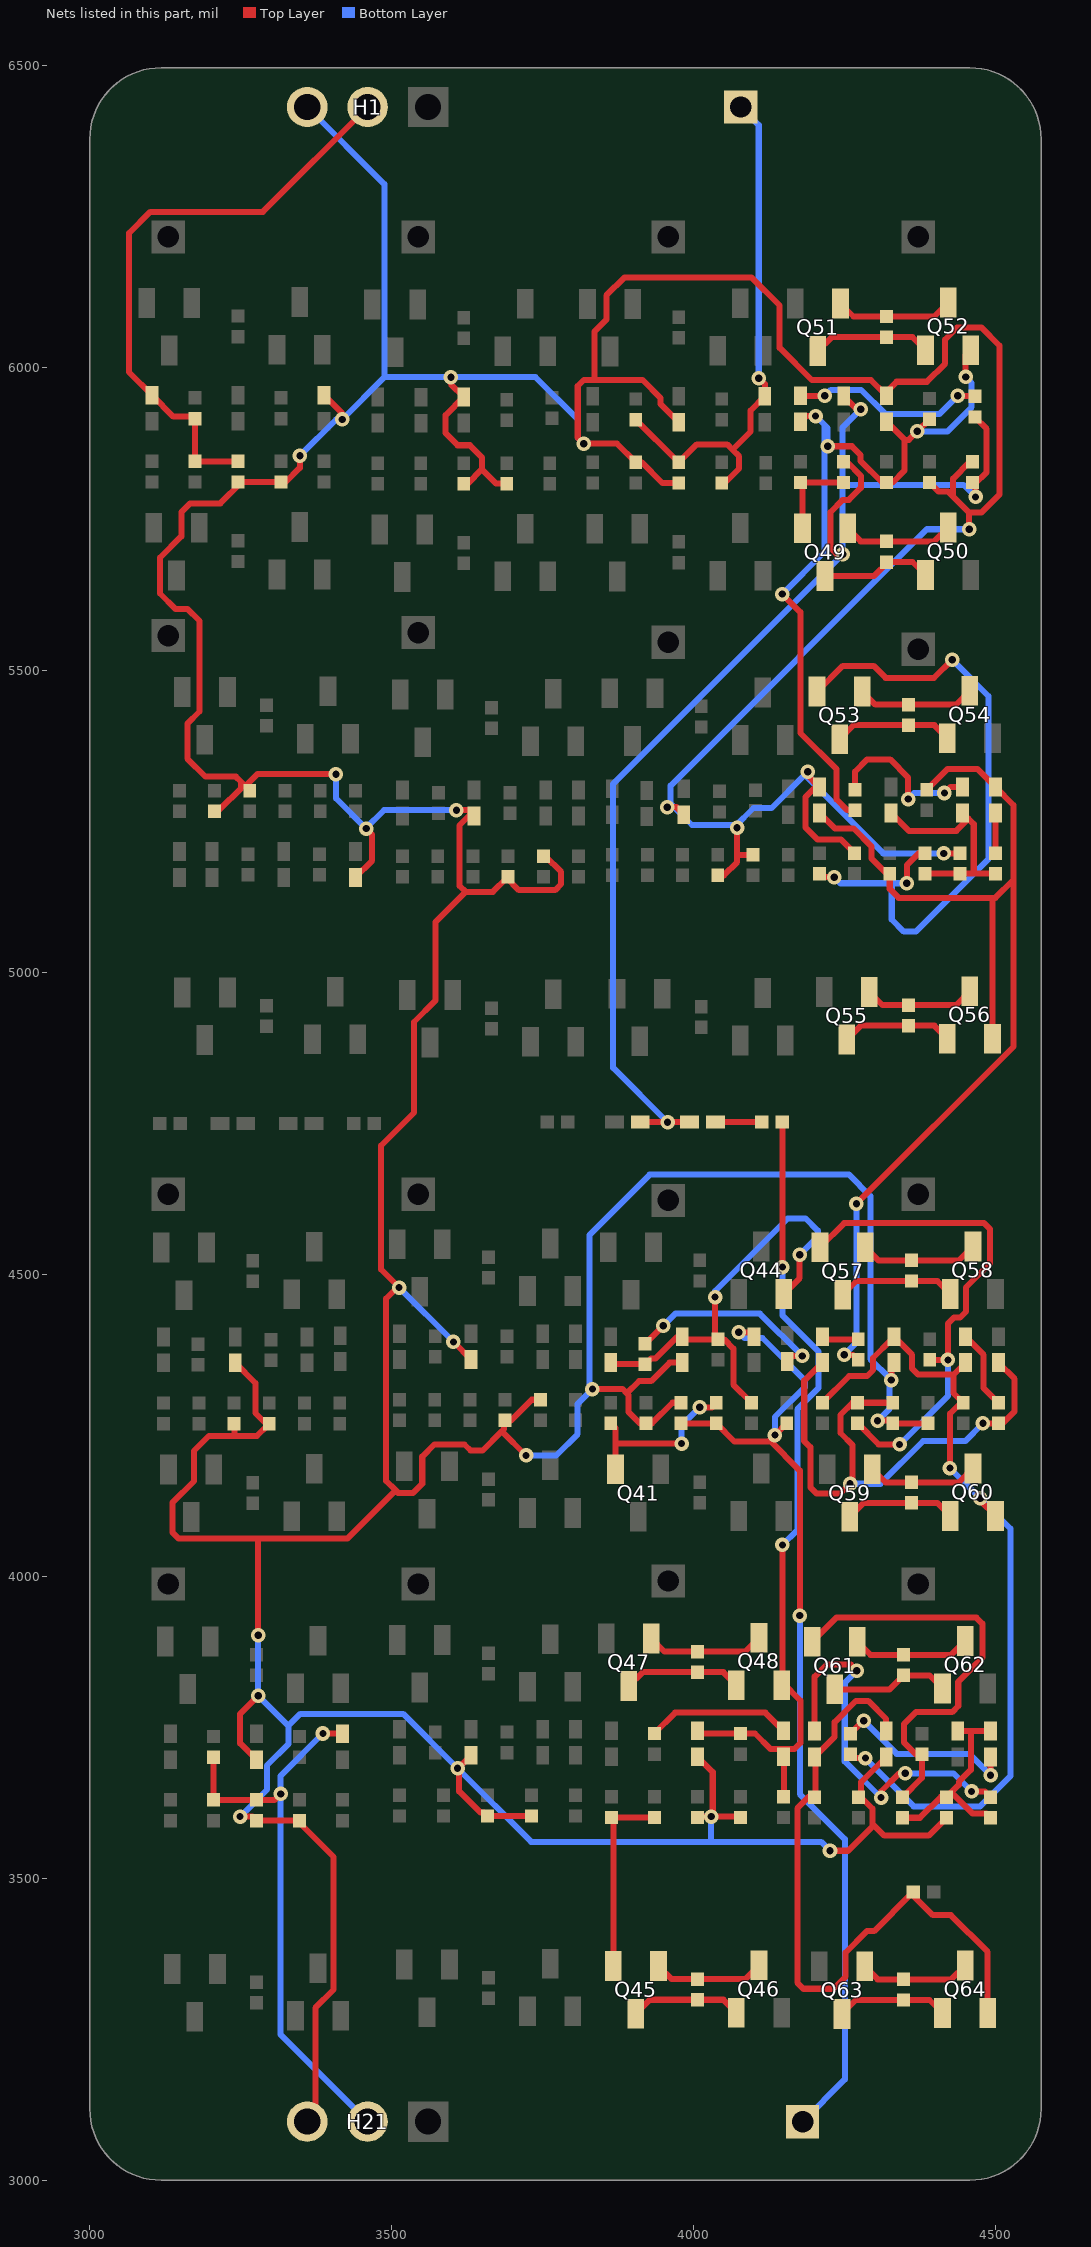
[diagram p0: the nets of this part, all layers, seen from the top]
# Altium PCB MISC61260.pcbdoc (part 3 of 4)
Units mil, origin at the board's own origin, x right, y up, seen from the top; angles counter-clockwise.
Board outline 1574.8 x 3497.01 mil, 2 copper layers (Top Layer, Bottom Layer), stack 62.206 mil thick; 303 components, 159 nets, 654 pads, 177 vias.

## Via types
v1: diameter 24.02, hole 12, Top Layer to Bottom Layer, 177 vias

## Nets (pads, with @x,y where several pads share a name; then routed paths per layer and width w, separated by ;. In a path a pad name is that pad's centre, name@x,y a point inside that pad or via, vN(x,y) a via of type N, cw(c..) or ccw(c..) an arc to the next point about the centre after c; other vN are vias at no path point) (continued)
$1N11454: C44.2 R42.1 | length 338.2
  Top Layer w10: R42.1@3919.35,4384.53 v1(3949.35,4414.53) ; C44.2@4154.58,4355.55 4163.56,4364.53 v1(4179.35,4364.53)
  Bottom Layer w10: v1(3949.35,4414.53) 3969.35,4434.53 4109.35,4434.53 v1(4179.35,4364.53)
$1N11455: C42.1 C43.1 Q44.2 R42.2 R43.2 Rp22.1 | length 771.1
  Top Layer w10: C43.1@3862.33,4353.53 3864.49,4351.37 R42.2@3920.28,4351.37 ; R42.2@3919.35,4350.45 R42.2@3920.28,4351.37 ; C42.1@3980.89,4396.45 C42.1@3981.78,4395.57 ; v1(4035.17,4462.03) Rp22.1@4035.17,4392.03 ; R43.2@4095.45,4287.03 4065.45,4317.03 4065.45,4376.75 4050.17,4392.03 Rp22.1@4040.17,4392.03 Rp22.1@4035.17,4392.03 ; Q44.2@4148.98,4467 4175.17,4493.19 v1(4175.17,4532.03) ; R42.2@3920.28,4351.37 3929.11,4360.21 3936.42,4360.21 3971.78,4395.57 C42.1@3981.78,4395.57 ; C42.1@3981.78,4395.57 3985.31,4392.03 Rp22.1@4035.17,4392.03
  Bottom Layer w10: v1(4035.17,4462.03) 4035.17,4472.03 4155.17,4592.03 4185.17,4592.03 4205.17,4572.03 4205.17,4562.03 v1(4175.17,4532.03)
$1N11457: Q41.2 Rp21.2 Rs21.1 | length 291.6
  Top Layer w10: Rp21.2@3862.33,4252.95 3870.39,4244.89 3870.39,4219.51 ; Q41.2@3870.39,4177.01 3870.39,4219.51 ; v1(3979.65,4219.51) 3870.39,4219.51 ; v1(4009.65,4279.51) 4029.65,4279.51 Rs21.1@4037.17,4287.03
  Bottom Layer w10: v1(3979.65,4219.51) 3979.65,4249.51 v1(4009.65,4279.51)
$1N11459: Q45.3 Q46.1 Rb23.2 | length 184.9
  Top Layer w10: Q45.3@3904.06,3275.77 3927.08,3298.79 Rb23.2@4005.95,3298.79 4048.81,3298.79 Q46.1@4070.45,3277.15
$1N11460: Q45.1 Q46.3 Rb23.1 | length 184.9
  Top Layer w10: Q45.1@3941.46,3354.51 3963.1,3332.87 Rb23.1@4005.95,3332.87 4084.83,3332.87 Q46.3@4107.85,3355.89
$1N11461: Q45.2 Rp23.2 Rs23.1 | length 318.4
  Top Layer w10: Q45.2@3866.66,3354.51 3866.66,3597.39 Rp23.2@3863.6,3600.45 Rs23.1@3934.78,3600.45
$1N11462: Q47.3 Q48.1 Rb24.2 | length 196.8
  Top Layer w10: Q47.3@3892.15,3818.12 3915.17,3841.14 Rb24.2@4005.95,3841.14 4048.81,3841.14 Q48.1@4070.45,3819.5
$1N11463: Q47.1 Q48.3 Rb24.1 | length 196.8
  Top Layer w10: Q47.1@3929.55,3896.86 3951.19,3875.22 Rb24.1@4005.95,3875.22 4084.83,3875.22 Q48.3@4107.85,3898.24
$1N11464: C47.2 R45.1 | length 240.2
  Top Layer w10: R45.1@3934.78,3739.53 3969.2,3773.95 4118.31,3773.95 C47.2@4148.31,3743.95
$1N11466: C46.1 C47.1 Q48.2 R47.2 R48.2 Rp24.1 | length 1363
  Top Layer w10: C46.1@4005.95,3743.95 4010.37,3739.53 Rp24.1@4077.13,3739.53 4101.17,3739.53 4126.62,3714.09 C47.1@4149.12,3714.09 ; Q48.2@4145.25,3819.5 4146.62,3820.87 Q48.2@4146.62,3824.09 ; v1(4146.62,4051.59) Q48.2@4146.62,3824.09 ; v1(4146.62,4511.59) R48.2@4146.62,4751.59 ; R47.2@4148.31,3634.53 4149.12,3635.34 C47.1@4149.12,3701.84 ; C47.1@4148.31,3701.03 C47.1@4149.12,3701.84 ; Q48.2@4146.62,3824.09 4176.62,3794.09 4176.62,3724.09 4166.62,3714.09 C47.1@4149.12,3714.09 ; C47.1@4149.12,3701.84 C47.1@4149.12,3714.09
  Bottom Layer w10: v1(4146.62,4051.59) 4171.26,4076.23 4171.26,4276.23 4206.62,4311.59 4206.62,4371.59 4146.62,4431.59 v1(4146.62,4511.59)
$1N11467: C48.2 R48.1 | length 76.9
  Top Layer w10: C48.2@4035.65,4751.59 R48.1@4112.54,4751.59
$1N11468: C40.1 C48.1 C49.2 R49.2 R51.1 Rs25.2 | length 2096.7
  Top Layer w10: C40.1@3911.42,4751.59 v1(3956.42,4751.59) C48.1@3992.73,4751.59 ; v1(4246.42,5691.59) 4236.42,5691.59 4226.42,5701.59 4226.42,5761.59 4246.42,5781.59 4256.42,5781.59 4276.42,5801.59 4276.42,5821.59 4253.48,5844.53 Rs25.2@4247.91,5844.53 ; C49.2@4248.14,5953.47 4270.02,5931.59 v1(4276.42,5931.59) ; R51.1@4461.45,5810.45 R51.1@4464.66,5807.24 ; R49.2@4465.17,5918.87 4484.66,5899.38 4484.66,5827.24 R51.1@4464.66,5807.24 ; v1(4466.42,5786.59) 4466.42,5805.47 R51.1@4464.66,5807.24
  Bottom Layer w10: v1(3956.42,4751.59) 3866.42,4841.59 3866.42,5311.59 v1(4246.42,5691.59) 4246.42,5806.59 ; v1(4276.42,5931.59) 4246.42,5901.59 4246.42,5806.59 ; v1(4466.42,5786.59) 4446.42,5806.59 4246.42,5806.59
$1N11498: Q49.3 Q50.1 Rb25.2 | length 187.4
  Top Layer w10: Q49.3@4217.19,5655.77 4298.57,5655.77 Rb25.2@4321.59,5678.79 ; Rb25.2@4319.09,5678.79 Rb25.2@4321.59,5678.79 ; Q50.1@4383.59,5657.15 4361.95,5678.79 Rb25.2@4321.59,5678.79
$1N11499: Q49.1 Q50.3 Rb25.1 | length 184.9
  Top Layer w10: Q49.1@4254.59,5734.51 4276.23,5712.87 Rb25.1@4319.09,5712.87 4397.97,5712.87 Q50.3@4420.99,5735.89
$1N11500: Q51.3 Q52.1 Rb26.2 | length 196.8
  Top Layer w10: Q51.3@4205.29,6028.12 4228.31,6051.14 Rb26.2@4319.09,6051.14 4361.95,6051.14 Q52.1@4383.59,6029.5
$1N11501: Q51.1 Q52.3 Rb26.1 | length 196.8
  Top Layer w10: Q51.1@4242.69,6106.86 4264.33,6085.22 Rb26.1@4319.09,6085.22 4397.97,6085.22 Q52.3@4420.99,6108.24
$1N11502: C51.2 R49.1 | length 322
  Top Layer w10: C51.2@4176.74,5953.95 v1(4216.74,5953.95) ; v1(4436.74,5953.95) 4464.17,5953.95 R49.1@4465.17,5952.95
  Bottom Layer w10: v1(4216.74,5953.95) 4226.74,5963.95 4276.74,5963.95 4316.74,5923.95 4406.74,5923.95 v1(4436.74,5953.95)
$1N11503: C50.1 C51.1 Q52.2 R50.2 R52.2 Rp26.1 | length 1334.9
  Top Layer w10: v1(4146.29,5625.75) 4176.29,5595.75 4176.29,5395.75 4236.29,5335.75 4236.29,5285.75 4254.09,5267.95 R52.2@4267.03,5267.95 ; C51.1@4176.74,5911.03 4186.16,5920.45 v1(4201.59,5920.45) ; v1(4221.59,5870.45) 4261.59,5870.45 4276.24,5855.81 4276.24,5845.81 4311.59,5810.45 R50.2@4319.09,5810.45 4329.09,5810.45 4349.09,5830.45 4349.09,5881.03 ; C50.1@4319.09,5911.03 4349.09,5881.03 ; Rp26.1@4390.27,5915.45 v1(4369.99,5895.17) 4355.85,5881.03 4349.09,5881.03 ; v1(4449.99,5985.17) 4449.99,6021.1 Q52.2@4458.39,6029.5
  Bottom Layer w10: v1(4146.29,5625.75) 4216.29,5695.75 4216.29,5905.75 ; v1(4201.59,5920.45) 4216.29,5905.75 ; v1(4221.59,5870.45) 4221.59,5900.45 4216.29,5905.75 ; v1(4369.99,5895.17) 4419.99,5895.17 4459.99,5935.17 4459.99,5975.17 v1(4449.99,5985.17)
$1N11512: Q49.2 Rp25.2 Rs25.1 | length 148.4
  Top Layer w10: Q49.2@4179.79,5734.51 4179.79,5807.39 Rp25.2@4176.74,5810.45 Rs25.1@4247.91,5810.45
$1N11514: C52.1 C53.2 R53.2 R54.1 Rs27.2 | length 373.6
  Top Layer w10: C53.2@4326.31,5263.53 4355.97,5233.87 4434.54,5233.87 C52.1@4454.54,5253.87 ; Rs27.2@4382.59,5162.95 R54.1@4440.87,5162.95 4463.37,5162.95 ; C52.1@4444.87,5263.53 C52.1@4454.54,5253.87 ; R53.2@4499.15,5162.95 4463.37,5162.95 ; C52.1@4454.54,5253.87 4463.37,5245.03 4463.37,5162.95
$1N11521: C52.2 R52.1 | length 272.4
  Top Layer w10: R52.1@4267.03,5302.03 4267.03,5332.03 4287.03,5352.03 4324.87,5352.03 4354.87,5322.03 v1(4354.87,5286.45) ; v1(4414.87,5296.45) 4424.87,5306.45 C52.2@4444.87,5306.45
  Bottom Layer w10: v1(4354.87,5286.45) 4364.87,5296.45 v1(4414.87,5296.45)
$1N11522: Q53.3 Q54.1 Rb27.2 | length 196.8
  Top Layer w10: Q53.3@4241.3,5385.62 4264.32,5408.64 Rb27.2@4355.11,5408.64 4397.97,5408.64 Q54.1@4419.61,5387
$1N11523: Q53.1 Q54.3 Rb27.1 | length 196.8
  Top Layer w10: Q53.1@4278.7,5464.36 4300.34,5442.72 Rb27.1@4355.11,5442.72 4433.99,5442.72 Q54.3@4457.01,5465.74
$1N11524: Q53.2 Rp27.2 Rs27.1 | length 1114.6
  Top Layer w10: Q53.2@4203.9,5464.36 4246.57,5507.03 4297.59,5507.03 4317.59,5487.03 4397.59,5487.03 v1(4427.59,5517.03) ; Rp27.2@4207.75,5162.95 4213.67,5157.03 v1(4232.59,5157.03) ; v1(4352.59,5147.03) 4352.59,5177.03 4372.59,5197.03 Rs27.1@4382.59,5197.03
  Bottom Layer w10: v1(4232.59,5157.03) 4242.59,5147.03 4327.59,5147.03 ; v1(4352.59,5147.03) 4327.59,5147.03 ; v1(4427.59,5517.03) 4487.59,5457.03 4487.59,5187.03 4367.59,5067.03 4347.59,5067.03 4327.59,5087.03 4327.59,5147.03
$1N11525: Q55.3 Q56.1 Rb28.2 | length 184.9
  Top Layer w10: Q55.3@4253.21,4888.27 4276.23,4911.29 Rb28.2@4355.11,4911.29 4397.97,4911.29 Q56.1@4419.61,4889.65
$1N11526: Q55.1 Q56.3 Rb28.1 | length 184.9
  Top Layer w10: Q55.1@4290.61,4967.01 4312.25,4945.37 Rb28.1@4355.11,4945.37 4433.99,4945.37 Q56.3@4457.01,4968.39
$1N11527: C55.2 R53.1 | length 66.5
  Top Layer w10: R53.1@4499.15,5197.03 C55.2@4499.15,5263.53
$1N11534: C54.1 C55.1 Q56.2 R55.2 R56.2 Rp28.1 | length 1888.7
  Top Layer w10: C54.1@4207.75,5263.53 4233.49,5237.79 4264.31,5237.79 4294.31,5207.79 4294.31,5187.79 R55.2@4324.31,5157.79 ; v1(4249.15,4366.45) 4263.53,4366.45 R56.2@4272.03,4357.95 ; v1(4269.15,4616.45) 4529.15,4876.45 4529.15,5152.95 ; R55.2@4324.31,5162.95 R55.2@4324.31,5157.79 ; Rp28.1@4385.59,5302.03 4420.01,5336.45 4469.15,5336.45 C55.1@4499.15,5306.45 4529.15,5276.45 4529.15,5152.95 ; Q56.2@4494.15,4889.91 4494.15,5122.95 ; R55.2@4324.31,5157.79 4324.31,5137.79 4339.15,5122.95 4494.15,5122.95 ; 4494.15,5122.95 4499.15,5122.95 4529.15,5152.95
  Bottom Layer w10: v1(4249.15,4366.45) 4269.15,4386.45 v1(4269.15,4616.45)
$1N11543: C56.1 C57.2 R57.2 R58.1 Rs29.2 | length 932.6
  Top Layer w10: C56.1@4212.75,4353.53 4182.75,4323.53 4182.75,4223.53 4192.75,4213.53 4192.75,4147.03 4202.75,4137.03 4242.75,4137.03 4262.75,4157.03 4262.75,4217.03 4242.75,4237.03 4242.75,4267.03 4262.75,4287.03 Rs29.2@4271.03,4287.03 R58.1@4329.31,4287.03 ; v1(4478.66,4252.94) 4511.16,4252.95 4531.16,4272.95 4531.16,4326.52 C57.2@4504.15,4353.53
  Bottom Layer w10: v1(4258.66,4152.94) 4308.66,4152.94 4379.37,4223.65 4449.37,4223.65 v1(4478.66,4252.94)
$1N11550: C56.2 R56.1 | length 61.1
  Top Layer w10: C56.2@4212.75,4396.45 4217.17,4392.03 R56.1@4272.03,4392.03
$1N11551: Q57.3 Q58.1 Rb29.2 | length 196.8
  Top Layer w10: Q57.3@4246.3,4465.62 4269.32,4488.64 Rb29.2@4360.11,4488.64 4402.97,4488.64 Q58.1@4424.61,4467
$1N11552: Q57.1 Q58.3 Rb29.1 | length 196.8
  Top Layer w10: Q57.1@4283.7,4544.36 4305.34,4522.72 Rb29.1@4360.11,4522.72 4438.99,4522.72 Q58.3@4462.01,4545.74
$1N11553: Q57.2 Rp29.2 Rs29.1 | length 840.9
  Top Layer w10: Q57.2@4208.9,4544.36 4248.9,4584.36 4480.59,4584.36 4490.59,4574.36 4490.59,4517.95 4450.59,4477.95 4450.59,4437.95 4440.59,4427.95 4430.59,4427.95 4420.59,4417.95 v1(4420.59,4357.95) Rp29.2@4390.59,4357.95 ; Rs29.1@4271.03,4252.95 4306.03,4217.95 v1(4340.59,4217.95)
  Bottom Layer w10: v1(4340.59,4217.95) 4420.59,4297.95 v1(4420.59,4357.95)
$1N11554: Q59.3 Q60.1 Rb30.2 | length 184.9
  Top Layer w10: Q59.3@4258.21,4098.27 4281.23,4121.29 Rb30.2@4360.11,4121.29 4402.97,4121.29 Q60.1@4424.61,4099.65
$1N11555: Q59.1 Q60.3 Rb30.1 | length 184.9
  Top Layer w10: Q59.1@4295.61,4177.01 4317.25,4155.37 Rb30.1@4360.11,4155.37 4438.99,4155.37 Q60.3@4462.01,4178.39
$1N11556: C59.2 R57.1 | length 131.9
  Top Layer w10: C59.2@4449.87,4396.45 4479.87,4366.45 4479.87,4311.31 R57.1@4504.15,4287.03
$1N11563: C58.1 C59.1 Q60.2 R59.2 R60.2 Rp30.1 | length 1428.9
  Top Layer w10: Rp30.1@4212.75,4287.03 4256.87,4331.15 4286.62,4331.15 4296.62,4341.15 4296.62,4361.15 4326.62,4391.15 C58.1@4336.62,4391.15 ; R60.2@4259.11,3705.03 4265.25,3698.89 v1(4284.02,3698.89) ; C58.1@4331.31,4396.45 C58.1@4336.62,4391.15 ; v1(4424.02,4178.89) 4424.02,4268.89 R59.2@4444.02,4288.89 ; R59.2@4445.87,4287.03 R59.2@4444.02,4288.89 ; C59.1@4449.87,4353.53 4429.87,4333.53 ; v1(4474.02,4128.89) 4474.02,4125.04 Q60.2@4499.41,4099.65 ; C58.1@4336.62,4391.15 4361.31,4366.45 4361.31,4343.53 4371.31,4333.53 4429.87,4333.53 ; 4429.87,4333.53 4429.87,4303.03 R59.2@4444.02,4288.89
  Bottom Layer w10: v1(4284.02,3698.89) 4364.02,3618.89 4474.02,3618.89 4524.02,3668.89 4524.02,4078.89 v1(4474.02,4128.89) v1(4424.02,4178.89)
$1N11572: C60.1 C61.2 R61.2 R62.1 Rs31.2 | length 351
  Top Layer w10: Rs31.2@4345.53,3600.03 4374.3,3600.03 4409.29,3635.01 R62.1@4419.29,3635.01 ; R62.1@4418.38,3634.11 R62.1@4419.29,3635.01 ; C61.2@4436.95,3743.53 4458.73,3743.53 ; R61.2@4491.23,3600.03 4484.53,3606.73 4461.71,3606.73 R62.1@4426.36,3642.08 ; C60.1@4491.23,3743.53 4458.73,3743.53 ; R62.1@4419.29,3635.01 R62.1@4426.36,3642.08 ; R62.1@4426.36,3642.08 4438.73,3654.46 4438.73,3659.46 4458.73,3679.46 4458.73,3743.53
$1N11579: C60.2 R60.1 | length 308.3
  Top Layer w10: R60.1@4259.11,3739.11 4280.61,3760.61 v1(4281.23,3760.61) ; v1(4491.23,3670.61) C60.2@4491.23,3700.61
  Bottom Layer w10: v1(4281.23,3760.61) 4335.88,3705.96 4455.88,3705.96 v1(4491.23,3670.61)
$1N11580: Q61.3 Q62.1 Rb31.2 | length 196.8
  Top Layer w10: Q61.3@4233.38,3812.7 4324.16,3812.7 Rb31.2@4347.18,3835.72 4390.04,3835.72 Q62.1@4411.68,3814.08
$1N11581: Q61.1 Q62.3 Rb31.1 | length 196.8
  Top Layer w10: Q61.1@4270.78,3891.44 4292.42,3869.8 Rb31.1@4347.18,3869.8 4426.06,3869.8 Q62.3@4449.08,3892.82
$1N11582: Q61.2 Rp31.2 Rs31.1 | length 710.3
  Top Layer w10: Q61.2@4195.98,3891.44 4235.98,3931.44 4467.67,3931.44 4477.67,3921.44 4477.67,3865.03 4437.67,3825.03 4437.67,3785.03 4427.67,3775.03 4367.67,3775.03 4347.67,3755.03 4347.67,3725.03 4367.67,3705.03 Rp31.2@4377.67,3705.03 4377.67,3666.25 Rs31.1@4345.53,3634.11
$1N11583: Q63.3 Q64.1 Rb32.2 | length 184.9
  Top Layer w10: Q63.3@4245.29,3275.35 4268.31,3298.37 Rb32.2@4347.18,3298.37 4390.04,3298.37 Q64.1@4411.68,3276.73
$1N11584: Q63.1 Q64.3 Rb32.1 | length 184.9
  Top Layer w10: Q63.1@4282.69,3354.09 4304.33,3332.45 Rb32.1@4347.18,3332.45 4426.06,3332.45 Q64.3@4449.08,3355.47
$1N11585: C63.2 R61.1 | length 635.7
  Top Layer w10: C63.2@4199.83,3743.53 4199.83,3833.53 4219.83,3853.53 4259.83,3853.53 v1(4269.83,3843.53) ; v1(4309.83,3633.53) 4309.83,3643.53 4339.83,3673.53 v1(4349.83,3673.53) ; v1(4459.83,3643.53) 4481.81,3643.53 R61.1@4491.23,3634.11
  Bottom Layer w10: v1(4269.83,3843.53) 4249.83,3823.53 4249.83,3693.53 v1(4309.83,3633.53) ; v1(4349.83,3673.53) 4429.83,3673.53 v1(4459.83,3643.53)
$1N16901: C62.1 C63.1 Q64.2 R63.2 Rp32.1 | length 1152
  Top Layer w10: Rp32.1@4199.83,3634.11 Rp32.1@4201.22,3635.49 ; C63.1@4199.83,3700.61 C63.1@4201.22,3701.99 ; C62.1@4318.39,3743.53 4318.39,3763.53 4288.39,3793.53 4268.39,3793.53 4233.04,3758.17 4233.04,3733.81 C63.1@4201.22,3701.99 ; R63.2@4362.96,3477.01 R63.2@4360.19,3474.24 ; Q64.2@4486.48,3276.73 4486.48,3377.94 4425.54,3438.88 4395.54,3438.88 R63.2@4360.19,3474.24 ; Rp32.1@4201.22,3635.49 C63.1@4201.22,3701.99 ; Rp32.1@4201.22,3635.49 4191.22,3635.49 4171.22,3615.49 4171.22,3327.01 4181.22,3317.01 4231.22,3317.01 4251.22,3337.01 4251.22,3377.01 4286.57,3412.36 4298.32,3412.36 R63.2@4360.19,3474.24
B1: C4.2 H1.2 R1.2 R3.1 Rs1.2 | length 995
  Top Layer w10: R3.1@3245.47,5845.38 Rs1.2@3174.29,5845.38 R1.2@3174.29,5916.3 3171.15,5919.45 3138.47,5919.45 C4.2@3103.12,5954.8 3064.88,5993.03 3064.88,6223.03 3100.24,6258.39 3286.38,6258.39 H1.2@3460,6432.01
B1': C10.2 H21.2 R11.2 R14.1 Rs5.2 | length 950
  Top Layer w10: R11.2@3204.78,3700.45 Rs5.2@3204.78,3629.53 R14.1@3275.95,3629.53 3305.95,3629.53 v1(3315.95,3639.53) ; v1(3385.95,3739.53) 3417.73,3739.53 C10.2@3418.31,3738.95
  Bottom Layer w10: v1(3385.95,3739.53) 3315.95,3669.53 v1(3315.95,3639.53) 3315.95,3241.05 H21.2@3460,3097.01
B2: C33.2 H20.1 R33.2 R36.1 Rs17.2 | length 888
  Top Layer w10: R33.2@3903.93,5914.6 3971.32,5847.22 R36.1@3978.64,5847.22 ; R36.1@3975.11,5843.69 R36.1@3978.64,5847.22 ; Rs17.2@4046.29,5809.6 4051.03,5809.6 4075.11,5833.69 4075.11,5853.69 4063.95,5864.85 ; v1(4107.46,5983.1) 4117.46,5973.1 C33.2@4117.46,5953.1 4093.95,5929.59 4093.95,5894.85 4063.95,5864.85 ; R36.1@3978.64,5847.22 4005.11,5873.69 4055.11,5873.69 4063.95,5864.85
  Bottom Layer w10: H20.1@4077.5,6432.01 4107.46,6402.05 v1(4107.46,5983.1)
B2': C41.2 H22.1 R41.2 R44.1 Rs21.2 | length 1689.9
  Top Layer w10: R44.1@3978.89,4252.95 Rs21.2@4037.17,4252.95 4067.17,4222.95 4123.73,4222.95 4125.5,4224.72 ; v1(4074.34,4403.56) 4092.34,4403.56 C41.2@4099.45,4396.45 ; R41.2@4153.73,4252.95 v1(4134.34,4233.56) 4125.5,4224.72 ; v1(4175.5,3934.72) 4175.5,4174.72 4125.5,4224.72
  Bottom Layer w10: v1(4074.34,4403.56) 4083.63,4394.27 4113.63,4394.27 4184.34,4323.56 4184.34,4313.56 4134.34,4263.56 v1(4134.34,4233.56) ; v1(4175.5,3934.72) 4175.5,3639.22 4250,3564.72 4250,3167.01 H22.1@4180,3097.01
GND: C5.2 C7.2 C11.2 C15.2 C19.2 C23.2 C27.2 C31.2 C34.2 C38.2 C42.2 C46.2 C50.2 C54.2 C58.2 C62.2 H1.3 H21.3 R3.2 R7.2 R14.2 R16.2 R21.2 R24.2 R28.2 R32.2 R36.2 R38.2 R44.2 R46.2 R51.2 R54.2 R58.2 R62.2 Rs2.2 Rs4.2 Rs6.2 Rs8.2 Rs10.2 Rs12.2 Rs14.2 Rs16.2 Rs18.2 Rs20.2 Rs22.2 Rs24.2 Rs26.2 Rs28.2 Rs30.2 Rs32.2 | length 14362.4
  Top Layer w10: R7.2@3206.63,5266.14 3209.77,5269.28 3215.13,5269.28 3250.49,5304.64 3250.49,5314.64 ; R16.2@3238.89,4252.53 3239.67,4251.75 3239.67,4232.04 ; C15.2@3240.89,4353.11 3274.36,4319.64 3274.36,4269.72 Rs8.2@3294.36,4249.72 ; R3.2@3245.47,5811.3 R3.2@3251.65,5811.3 ; v1(3248.77,3602.04) 3269.36,3602.04 R14.2@3275.95,3595.45 Rs6.2@3343.45,3595.45 ; Rs4.2@3264.91,5300.22 Rs4.2@3257.56,5307.57 ; C11.2@3275.95,3696.03 3248.77,3723.21 3248.77,3772.04 v1(3278.77,3802.04) ; v1(3278.77,3902.04) 3278.77,4062.04 ; Rs8.2@3297.17,4252.53 Rs8.2@3294.36,4249.72 ; Rs6.2@3347.13,3595.45 Rs6.2@3343.45,3595.45 ; v1(3347.83,5854.8) 3347.83,5834.8 3324.33,5811.3 Rs2.2@3316.65,5811.3 R3.2@3251.65,5811.3 ; H21.3@3360,3097.01 3373.45,3110.46 3373.45,3285.45 3403.45,3315.45 3403.45,3535.45 Rs6.2@3343.45,3595.45 ; C5.2@3387.83,5954.8 3417.83,5924.8 v1(3417.83,5914.8) ; v1(3407.56,5327.57) 3277.56,5327.57 Rs4.2@3257.56,5307.57 ; C7.2@3439.75,5156.72 3467.56,5184.53 3467.56,5227.57 v1(3457.56,5237.57) ; v1(3512.08,4477.77) v1@3510.36,4479.48 ; v1(3597.83,5984.8) 3597.83,5973.35 C19.2@3619.09,5952.09 3589.09,5922.09 3589.09,5892.09 3609.09,5872.09 3629.09,5872.09 3649.09,5852.09 3649.09,5832.09 ; v1(3602.08,4387.77) C27.2@3631.31,4358.53 ; v1(3607.06,5268.07) 3626.77,5268.07 C23.2@3632.08,5262.77 ; v1(3608.77,3682.04) 3609.82,3682.04 v1@3611.59,3683.81 ; R21.2@3619.09,5808.59 3625.59,5808.59 3649.09,5832.09 ; C31.2@3631.31,3703.53 v1@3611.59,3683.81 ; C23.2@3636.31,5258.53 C23.2@3632.08,5262.77 ; Rs10.2@3690.27,5808.59 3672.59,5808.59 3649.09,5832.09 ; Rs12.2@3692.59,5157.95 Rs12.2@3690.39,5155.75 ; v1(3722.18,4199.77) 3682.18,4239.77 ; R32.2@3731.3,3602.95 Rs16.2@3658.45,3602.95 3652.95,3608.45 3646.95,3608.45 3611.59,3643.81 v1@3611.59,3683.81 ; R28.2@3745.87,4292.03 3731.67,4292.03 3697.59,4257.95 Rs14.2@3687.59,4257.95 3685.72,4256.07 3685.72,4243.31 3682.18,4239.77 ; R24.2@3750.87,5192.03 3754.11,5192.03 3780.39,5165.75 3780.39,5145.75 3770.39,5135.75 3710.39,5135.75 Rs12.2@3690.39,5155.75 ; v1(3832.18,4309.77) 3882.18,4309.77 3889.25,4302.7 ; v1(3955.84,5273.06) 3970.94,5273.06 C38.2@3983.39,5260.61 ; R36.2@3975.11,5809.6 3948.01,5809.6 3913.93,5843.69 Rs18.2@3903.93,5843.69 3872.81,5874.8 v1(3817.83,5874.8) 3807.83,5884.8 3807.83,5970.19 3817.83,5980.19 3835.33,5980.19 ; C34.2@3975.11,5910.19 3945.11,5940.19 3945.11,5950.19 3915.11,5980.19 3835.33,5980.19 ; R44.2@3978.89,4287.03 3964.69,4287.03 3930.61,4252.95 Rs22.2@3920.61,4252.95 3910.61,4252.95 3892.18,4271.38 3892.18,4299.77 3889.25,4302.7 ; C42.2@3980.89,4353.53 3960.08,4353.53 3929.25,4322.7 3909.25,4322.7 3889.25,4302.7 ; R46.2@4005.95,3600.45 4007.54,3602.04 v1(4028.77,3602.04) v1@4031.27,3602.04 ; C46.2@4005.95,3701.03 4031.27,3675.71 v1@4031.27,3602.04 ; Rs20.2@4039.67,5160.03 4049.67,5160.03 4071.57,5181.93 4071.57,5193.79 ; v1(4071.57,5238.79) 4071.57,5193.79 ; Rs24.2@4077.13,3600.45 4075.54,3602.04 v1@4031.27,3602.04 ; R38.2@4097.95,5194.11 4097.63,5193.79 4071.57,5193.79 ; v1(4188.7,5331.67) 4188.7,5325.51 C54.2@4204.61,5309.6 ; C54.2@4207.75,5306.45 C54.2@4204.61,5309.6 ; v1(4225.39,3545.42) 4255.39,3545.42 4295.39,3585.42 4295.39,3590.42 ; Rs28.2@4266.03,5197.03 4243.47,5219.6 4204.61,5219.6 4184.61,5239.6 4184.61,5289.6 C54.2@4204.61,5309.6 ; Rs32.2@4272.68,3634.11 Rs32.2@4276.71,3634.11 ; v1(4304.16,4257.4) 4324.87,4257.4 R58.2@4329.31,4252.95 Rs30.2@4387.59,4252.95 ; C62.2@4318.39,3700.61 4276.71,3658.92 Rs32.2@4276.71,3634.11 ; C50.2@4319.09,5953.95 C50.2@4315.84,5957.2 ; v1(4326.98,4324.57) 4326.98,4349.2 C58.2@4331.31,4353.53 ; Rs26.2@4390.27,5810.45 4404.91,5795.81 4420.48,5795.81 4429.32,5786.97 ; v1(4413.5,5196.47) 4440.31,5196.47 R54.2@4440.87,5197.03 ; R62.2@4418.38,3600.03 4388.77,3570.42 4315.39,3570.42 4295.39,3590.42 ; v1(4455.84,5733.06) 4455.84,5760.45 ; R51.2@4461.45,5844.53 4456.89,5844.53 4429.32,5816.97 4429.32,5786.97 ; 3239.67,4232.04 3197.17,4232.04 3172.53,4207.4 3172.53,4157.4 3137.17,4122.04 3137.17,4072.04 3147.17,4062.04 3278.77,4062.04 ; 3239.67,4232.04 3276.68,4232.04 Rs8.2@3294.36,4249.72 ; 3250.49,5314.64 3241.65,5323.48 3191.65,5323.48 3161.65,5353.48 3161.65,5411.3 3181.65,5431.3 3181.65,5581.3 3161.65,5601.3 3141.65,5601.3 3116.29,5626.66 3116.29,5685.95 3151.65,5721.3 3151.65,5761.3 3166.29,5775.95 3216.29,5775.95 R3.2@3251.65,5811.3 ; 3250.49,5314.64 Rs4.2@3257.56,5307.57 ; 3278.77,4062.04 3426.27,4062.04 3506.27,4142.04 ; 3506.27,4142.04 3490.36,4157.95 3490.36,4459.48 v1@3510.36,4479.48 ; 3506.27,4142.04 3510.36,4137.95 3535.36,4137.95 3550.36,4152.95 3550.36,4197.95 3570.36,4217.95 3620.36,4217.95 3630.36,4207.95 3650.36,4207.95 3682.18,4239.77 ; v1@3510.36,4479.48 3482.08,4507.77 3482.08,4712.77 3536.72,4767.41 3536.72,4917.41 3572.08,4952.77 3572.08,5082.77 3622.08,5132.77 ; 3622.08,5132.77 3612.08,5142.77 3612.08,5242.77 C23.2@3632.08,5262.77 ; 3622.08,5132.77 3667.41,5132.77 Rs12.2@3690.39,5155.75 ; 3835.33,5980.19 3835.33,6060.19 3855.33,6080.19 3855.33,6120.19 3885.33,6150.19 4095.33,6150.19 4142.07,6103.44 4142.07,6033.44 4195.33,5980.19 4292.86,5980.19 C50.2@4315.84,5957.2 ; Rs32.2@4276.71,3634.11 4295.39,3615.42 4295.39,3590.42 ; C50.2@4315.84,5957.2 4335.84,5977.2 4385.84,5977.2 4415.84,6007.2 4415.84,6047.2 4435.84,6067.2 4475.84,6067.2 4505.84,6037.2 4505.84,5790.45 4475.84,5760.45 4455.84,5760.45 ; 4429.32,5786.97 4455.84,5760.45
  Bottom Layer w10: v1(3248.77,3602.04) 3293.42,3646.69 3293.42,3686.69 3328.77,3722.04 3328.77,3752.04 ; v1(3278.77,3902.04) v1(3278.77,3802.04) 3328.77,3752.04 ; v1(3347.83,5854.8) 3407.83,5914.8 v1(3417.83,5914.8) 3487.83,5984.8 ; H1.3@3360,6432.01 3487.83,6304.18 3487.83,5984.8 ; v1(3407.56,5327.57) 3407.56,5287.57 v1@3457.06,5238.07 ; v1(3457.56,5237.57) v1@3457.06,5238.07 ; v1(3512.08,4477.77) v1(3602.08,4387.77) ; v1(3607.06,5268.07) 3487.06,5268.07 v1@3457.06,5238.07 ; v1(3722.18,4199.77) 3772.18,4199.77 3807.54,4235.13 3807.54,4285.13 v1@3826.98,4304.57 ; v1(3817.83,5874.8) 3808.54,5884.09 3808.54,5914.09 3737.83,5984.8 v1(3597.83,5984.8) 3487.83,5984.8 ; v1(3832.18,4309.77) v1@3826.98,4304.57 ; v1(3955.84,5273.06) v1@3961.57,5278.79 ; v1(4028.77,3602.04) 4028.77,3561.71 4027.13,3560.07 ; v1(4071.57,5238.79) v1@4068.7,5241.67 ; v1(4188.7,5331.67) v1@4183.5,5326.47 ; v1(4225.39,3545.42) 4210.75,3560.07 4027.13,3560.07 ; v1(4304.16,4257.4) 4324.16,4277.4 v1@4324.16,4327.4 ; v1(4326.98,4324.57) v1@4324.16,4327.4 ; v1(4413.5,5196.47) 4313.5,5196.47 v1@4183.5,5326.47 ; v1(4455.84,5733.06) 4385.84,5733.06 3961.57,5308.79 v1@3961.57,5278.79 ; 3328.77,3752.04 3348.77,3772.04 3518.77,3772.04 v1(3608.77,3682.04) 3730.75,3560.07 4027.13,3560.07 ; v1@3826.98,4304.57 3826.98,4564.57 3926.98,4664.57 4256.98,4664.57 4292.34,4629.22 4292.34,4359.22 v1@4324.16,4327.4 ; v1@3961.57,5278.79 3996.93,5243.44 4066.93,5243.44 v1@4068.7,5241.67 ; v1@4068.7,5241.67 4098.7,5271.67 4128.7,5271.67 v1@4183.5,5326.47